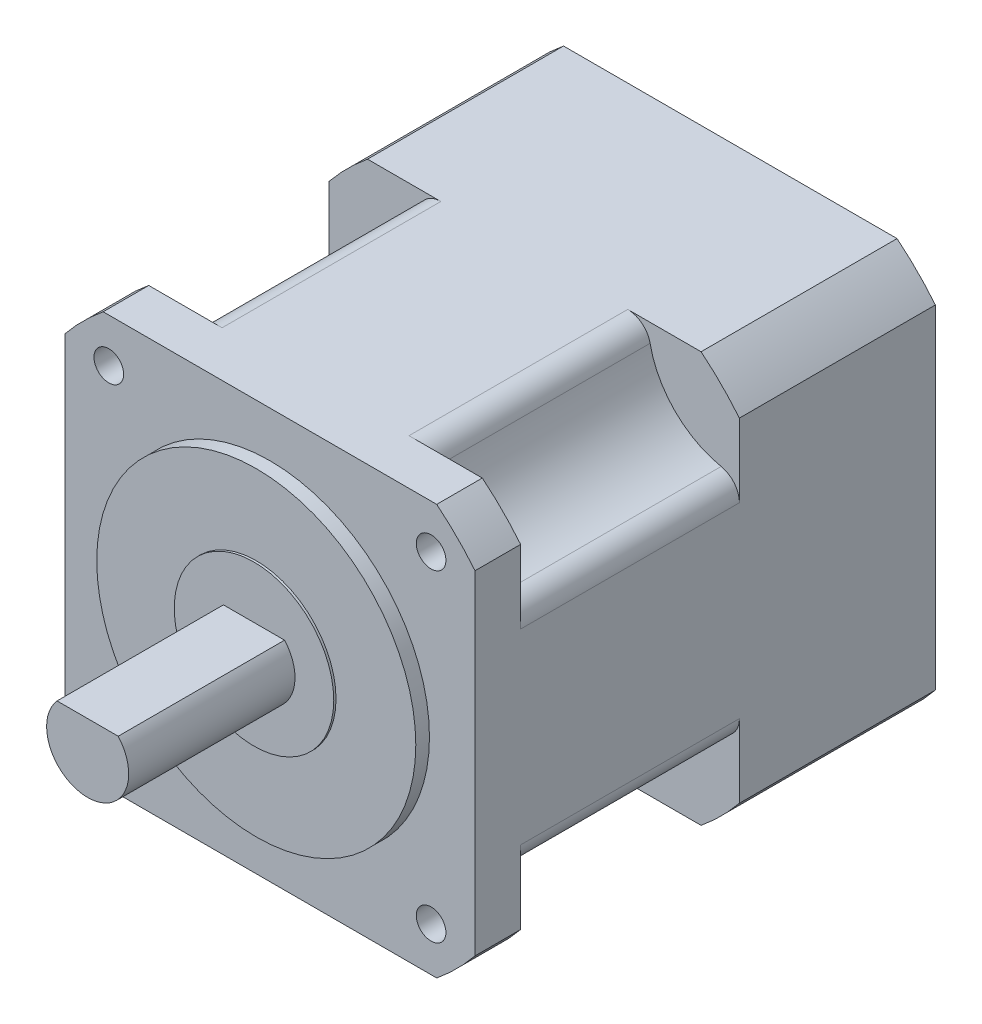
SolidWorks part; units mm, degrees
ref_plane "前视" through (0, 0, 0) normal (0, 0, 1) x (1, 0, 0)
ref_plane "上视" through (0, 0, 0) normal (0, 1, 0) x (1, 0, 0)
ref_plane "右视" through (0, 0, 0) normal (1, 0, 0) x (0, 0, -1)
sketch "草图1" plane through (0, 0, 0) normal (0, 0, 1) x (1, 0, 0)
  line L1 (0, 0) -> (90, 0)
  line L2 (0, 0) -> (0, 90)
  line L3 (0, 90) -> (90, 90)
  line L4 (90, 0) -> (90, 90)
  dimension "D1" = 90
  dimension "D2" = 90
extrude "拉伸1" add sketch "草图1" along normal blind 10
sketch "草图2" plane through (0, 0, 10) normal (0, 0, 1) x (1, 0, 0)
  line L0 (0, 45) -> (90, 45) construction
  line L1 (0, 90) -> (0, 0) construction
  line L2 (90, 0) -> (90, 90) construction
  line L3 (45, 90) -> (45, 0) construction
  line L4 (90, 90) -> (0, 90) construction
  line L5 (0, 0) -> (90, 0) construction
  circle A0 centre (45, 45) radius 35
  dimension "D1" = 70
extrude "拉伸2" add sketch "草图2" along normal blind 3
sketch "草图3" plane through (0, 0, 13) normal (0, 0, 1) x (1, 0, 0)
  circle A0 centre (45, 45) radius 17.5
  circle A1 centre (45, 45) radius 35 construction
  dimension "D1" = 35
extrude "拉伸3" add sketch "草图3" along normal blind 0.5
sketch "草图4" plane through (0, 0, 13.5) normal (0, 0, 1) x (1, 0, 0)
  line L0 (38.2918, 51) -> (51.7082, 51)
  arc A0 (38.2918, 51) -> (51.7082, 51) centre (45, 45) ccw
  circle A1 centre (45, 45) radius 17.5 construction
  dimension "D1" = 18
  dimension "D2" = 6
extrude "拉伸4" add sketch "草图4" along normal blind 36.5
sketch "草图5" plane through (0, 0, 10) normal (0, 0, 1) x (1, 0, 0)
  line L0 (0, 45) -> (90, 45) construction
  line L1 (0, 90) -> (0, 0) construction
  line L2 (90, 0) -> (90, 90) construction
  line L3 (45, 90) -> (45, 0) construction
  line L4 (90, 90) -> (0, 90) construction
  line L5 (0, 0) -> (90, 0) construction
  line L6 (0, 90) -> (90, 0) construction
  line L7 (90, 90) -> (0, 0) construction
  circle A0 centre (9.6447, 80.3553) radius 3.25
  circle A1 centre (80.3553, 80.3553) radius 3.25
  circle A2 centre (80.3553, 9.6447) radius 3.25
  circle A3 centre (9.6447, 9.6447) radius 3.25
  dimension "D1" = 6.5
  dimension "D2" = 50
extrude "切除-拉伸1" cut sketch "草图5" against normal up to next
sketch "草图6" plane through (0, 0, 10) normal (0, 0, 1) x (1, 0, 0)
  circle A0 centre (45, 45) radius 58
  circle A2 centre (45, 45) radius 35 construction
  dimension "D1" = 116
sketch "草图7" plane through (0, 0, 0) normal (0, 0, -1) x (-1, 0, 0)
  line L1 (-90, 90) -> (0, 90)
  line L2 (-90, 90) -> (-90, 0)
  line L3 (-90, 0) -> (0, 0)
  line L4 (0, 90) -> (0, 0)
extrude "拉伸5" add sketch "草图7" along normal blind 91
sketch "草图8" plane through (0, 0, 0) normal (0, 0, 1) x (1, 0, 0)
  line L0 (45, 90) -> (45, 0) construction
  line L3 (90, 90) -> (0, 90) construction
  line L4 (0, 0) -> (90, 0) construction
  line L5 (0, 45) -> (90, 45) construction
  line L6 (0, 90) -> (0, 0) construction
  line L7 (90, 0) -> (90, 90) construction
  circle A0 centre (90, 90) radius 20
  circle A2 centre (90, 0) radius 20
  circle A3 centre (0, 0) radius 20
  circle A4 centre (0, 90) radius 20
  dimension "D1" = 40
extrude "切除-拉伸2" cut sketch "草图8" against normal blind 48
fillet "圆角1" radius 5 8 edges at (70, 0, -24) (20, 0, -24) (0, 20, -24) (0, 70, -24) (20, 90, -24) (90, 20, -24) (90, 70, -24) (70, 90, -24)
extrude "切除-拉伸3" cut sketch "草图6" against normal through all flip side to cut
